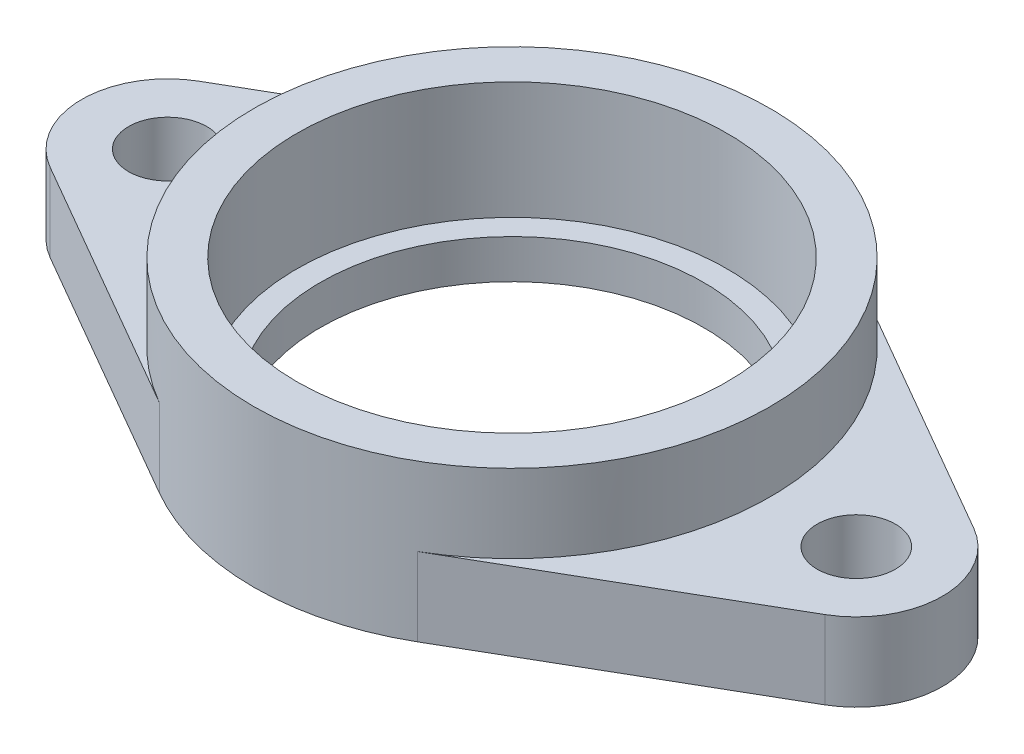
from build123d import *

# Parameters (mm, degrees)
SKETCH_1_R          = 5
EXTRUDE_1_DEPTH     = 10
SKETCH_2_R          = 33
EXTRUDE_2_DEPTH     = 10
SKETCH_3_R          = 27.5
CUT_EXTRUDE_1_DEPTH = 15
SKETCH_4_R          = 24.5
CUT_EXTRUDE_2_DEPTH = 15


with BuildPart() as part:
    # 草图1 → 凸台-拉伸1 (new body)
    with BuildSketch(Plane(origin=(0, 0, 0), x_dir=(1, 0, 0), z_dir=(0, 1, 0))):
        with BuildLine():
            Line((-49.5, 9.526279442), (-16.5, 28.578838325))
            ThreePointArc((-16.5, 28.578838325), (0, 33), (16.5, 28.578838325))
            Line((16.5, 28.578838325), (49.5, 9.526279442))
            ThreePointArc((49.5, 9.526279442), (55, 0), (49.5, -9.526279442))
            Line((49.5, -9.526279442), (16.5, -28.578838325))
            ThreePointArc((16.5, -28.578838325), (0, -33), (-16.5, -28.578838325))
            Line((-16.5, -28.578838325), (-49.5, -9.526279442))
            ThreePointArc((-49.5, -9.526279442), (-55, 0), (-49.5, 9.526279442))
        make_face()
        with Locations(Location((-44, 0, 0), (0, 0, 270))):
            Circle(SKETCH_1_R, mode=Mode.SUBTRACT)
        with Locations(Location((44, 0, 0), (0, 0, 270))):
            Circle(SKETCH_1_R, mode=Mode.SUBTRACT)
    extrude(amount=EXTRUDE_1_DEPTH)

    # 草图2 → 凸台-拉伸2 (add)
    with BuildSketch(Plane(origin=(0, 10, 0), x_dir=(1, 0, 0), z_dir=(0, 1, 0))):
        with Locations(Location((0, 0, 0), (0, 0, 120))):
            Circle(SKETCH_2_R)
    extrude(amount=EXTRUDE_2_DEPTH)

    # 草图3 → 切除-拉伸1 (cut)
    with BuildSketch(Plane(origin=(0, 20, 0), x_dir=(1, 0, 0), z_dir=(0, 1, 0))):
        with Locations(Location((0, 0, 0), (0, 0, 270))):
            Circle(SKETCH_3_R)
    extrude(amount=-CUT_EXTRUDE_1_DEPTH, mode=Mode.SUBTRACT)

    # 草图4 → 切除-拉伸2 (cut)
    with BuildSketch(Plane(origin=(0, 5, 0), x_dir=(1, 0, 0), z_dir=(0, 1, 0))):
        with Locations(Location((0, 0, 0), (0, 0, 270))):
            Circle(SKETCH_4_R)
    extrude(amount=-CUT_EXTRUDE_2_DEPTH, mode=Mode.SUBTRACT)


solid = part.part
